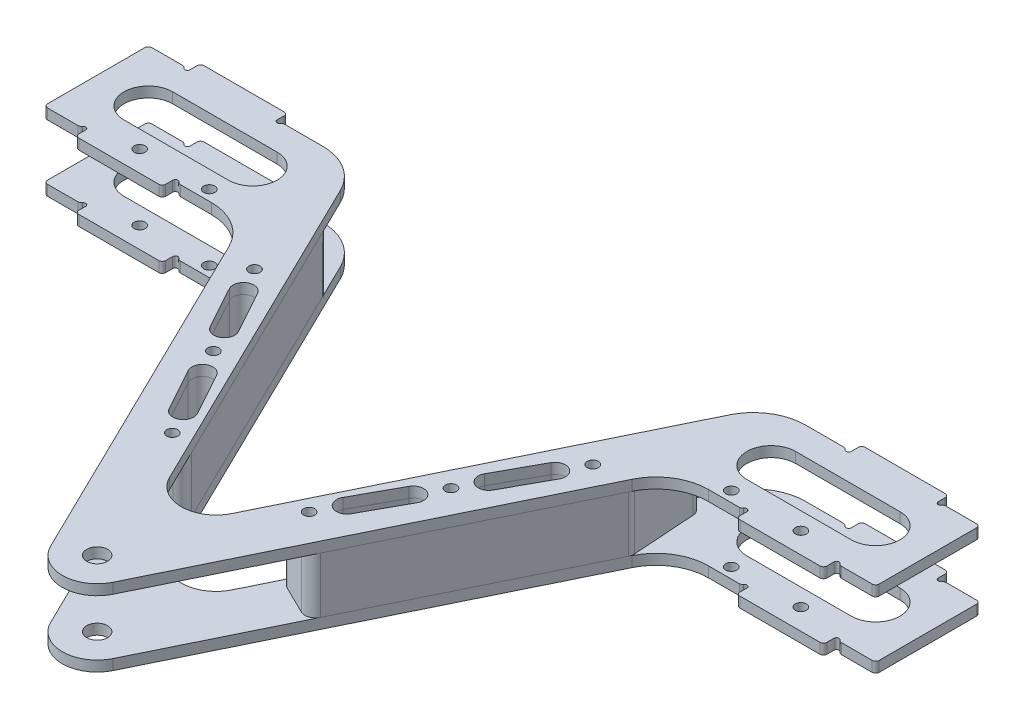
from build123d import *

# Parameters (mm, degrees)
SKETCH_1_R          = 3
EXTRUDE_1_DEPTH     = 3
SKETCH_2_R          = 0.75
CUT_EXTRUDE_1_DEPTH = 3
FILLET_1_R          = 1
EXTRUDE_2_DEPTH     = 16
EXTRUDE_2_2_DEPTH   = 16
SKETCH_4_R          = 1.6
CUT_EXTRUDE_2_DEPTH = 201.908561291
SKETCH_5_R          = 1.6
CUT_EXTRUDE_3_DEPTH = 201.908561291
CUT_EXTRUDE_4_DEPTH = 201.908561291


with BuildPart() as part:
    # 草图1 → 凸台-拉伸1 (new body)
    with BuildSketch(Plane(origin=(0, 0, 0), x_dir=(1, 0, 0), z_dir=(0, 1, 0))):
        with BuildLine():
            Line((-107.5, 127), (-107.5, 124))
            Line((-107.5, 124), (-82.5, 124))
            Line((-82.5, 124), (-82.5, 127))
            Line((-82.5, 127), (-71.405746163, 127))
            ThreePointArc((-71.405746163, 127), (-63.460885028, 124.723174979), (-57.927898376, 118.583890874))
            Line((-57.927898376, 118.583890874), (-8.985231858, 18.393620069))
            ThreePointArc((-8.985231858, 18.393620069), (0, 12.782880651), (8.985231858, 18.393620069))
            Line((8.985231858, 18.393620069), (57.927898376, 118.583890874))
            ThreePointArc((57.927898376, 118.583890874), (63.460885028, 124.723174979), (71.405746163, 127))
            Line((71.405746163, 127), (82.5, 127))
            Line((82.5, 127), (82.5, 124))
            Line((82.5, 124), (107.5, 124))
            Line((107.5, 124), (107.5, 127))
            Line((107.5, 127), (119.5, 127))
            Line((119.5, 127), (119.5, 157))
            Line((119.5, 157), (107.5, 157))
            Line((107.5, 157), (107.5, 160))
            Line((107.5, 160), (82.5, 160))
            Line((82.5, 160), (82.5, 157))
            Line((82.5, 157), (69.366602064, 157))
            ThreePointArc((69.366602064, 157), (61.421740929, 154.723174979), (55.888754277, 148.583890874))
            Line((55.888754277, 148.583890874), (8.985231858, 52.567941045))
            ThreePointArc((8.985231858, 52.567941045), (0, 46.957201628), (-8.985231858, 52.567941045))
            Line((-8.985231858, 52.567941045), (-55.888754277, 148.583890874))
            ThreePointArc((-55.888754277, 148.583890874), (-61.421740929, 154.723174979), (-69.366602064, 157))
            Line((-69.366602064, 157), (-82.5, 157))
            Line((-82.5, 157), (-82.5, 160))
            Line((-82.5, 160), (-107.5, 160))
            Line((-107.5, 160), (-107.5, 157))
            Line((-107.5, 157), (-119.5, 157))
            Line((-119.5, 157), (-119.5, 127))
            Line((-119.5, 127), (-107.5, 127))
        make_face()
        with Locations(Location((0, 22.782880651, 0), (0, 0, 270))):
            Circle(SKETCH_1_R, mode=Mode.SUBTRACT)
    extrude(amount=EXTRUDE_1_DEPTH)

    # 草图2 → 切除-拉伸1 (cut)
    with BuildSketch(Plane(origin=(0, 3, 0), x_dir=(1, 0, 0), z_dir=(0, 1, 0))):
        with Locations((-108.25, 157)):
            Circle(SKETCH_2_R)
        with Locations((-81.75, 157)):
            Circle(SKETCH_2_R)
        with Locations((-108.25, 127)):
            Circle(SKETCH_2_R)
        with Locations((-81.75, 127)):
            Circle(SKETCH_2_R)
        with Locations((81.75, 127)):
            Circle(SKETCH_2_R)
        with Locations((108.25, 127)):
            Circle(SKETCH_2_R)
        with Locations((81.75, 157)):
            Circle(SKETCH_2_R)
        with Locations((108.25, 157)):
            Circle(SKETCH_2_R)
    extrude(amount=-CUT_EXTRUDE_1_DEPTH, mode=Mode.SUBTRACT)

    # 圆角1
    fillet_1_edges = [part.edges().sort_by_distance(p)[0] for p in [
        (81, 1.5, -157),
        (109, 1.5, -127),
        (-81, 1.5, -127),
        (81, 1.5, -127),
        (-109, 1.5, -127),
        (-81, 1.5, -157),
        (109, 1.5, -157),
        (-119.5, 1.5, -127),
        (-119.5, 1.5, -157),
        (-107.5, 1.5, -160),
        (-82.5, 1.5, -160),
        (82.5, 1.5, -160),
        (107.5, 1.5, -160),
        (119.5, 1.5, -157),
        (119.5, 1.5, -127),
        (107.5, 1.5, -124),
        (82.5, 1.5, -124),
        (-82.5, 1.5, -124),
        (-107.5, 1.5, -124),
        (-109, 1.5, -157),
    ]]
    fillet(fillet_1_edges, radius=FILLET_1_R)


with BuildPart() as body_2:
    # 草图3 → 凸台-拉伸2 (new body)
    with BuildSketch(Plane(origin=(0, 3, 0), x_dir=(1, 0, 0), z_dir=(0, 1, 0))):
        with BuildLine():
            Line((-56.650043824, 137.383757235), (-57.873530284, 119.383757235))
            ThreePointArc((-57.873530284, 119.383757235), (-57.824581944, 118.604111022), (-57.576006101, 117.863534079))
            Line((-57.576006101, 117.863534079), (-28.519852473, 58.382837427))
            ThreePointArc((-28.519852473, 58.382837427), (-26.799235652, 56.862457312), (-24.507504741, 57.004046044))
            Line((-24.507504741, 57.004046044), (-16.420796069, 60.954380569))
            ThreePointArc((-16.420796069, 60.954380569), (-14.900415954, 62.674997389), (-15.042004686, 64.966728301))
            Line((-15.042004686, 64.966728301), (-50.961380526, 138.497090429))
            ThreePointArc((-50.961380526, 138.497090429), (-54.233151316, 140.124457655), (-56.650043824, 137.383757235))
        make_face()
    extrude(amount=EXTRUDE_2_DEPTH)


with BuildPart() as body_3:
    # 草图3 → Extrude 2 2 (new body)
    with BuildSketch(Plane(origin=(0, 3, 0), x_dir=(1, 0, 0), z_dir=(0, 1, 0))):
        with BuildLine():
            Line((56.650043824, 137.383757235), (57.873530284, 119.383757235))
            ThreePointArc((57.873530284, 119.383757235), (57.824581944, 118.604111022), (57.576006101, 117.863534079))
            Line((57.576006101, 117.863534079), (28.519852473, 58.382837427))
            ThreePointArc((28.519852473, 58.382837427), (26.799235652, 56.862457312), (24.507504741, 57.004046044))
            Line((24.507504741, 57.004046044), (16.420796069, 60.954380569))
            ThreePointArc((16.420796069, 60.954380569), (14.900415954, 62.674997389), (15.042004686, 64.966728301))
            Line((15.042004686, 64.966728301), (50.961380526, 138.497090429))
            ThreePointArc((50.961380526, 138.497090429), (54.233151316, 140.124457655), (56.650043824, 137.383757235))
        make_face()
    extrude(amount=EXTRUDE_2_2_DEPTH)


with BuildPart() as body_4:
    # 镜向1: mirrored copy
    add(part.part.mirror(Plane.ZX.offset(11)))


with BuildPart() as cut_extrude_2_tool:
    # 草图4 → 切除-拉伸2 (new, through all)
    with BuildSketch(Plane(origin=(0, 22, 0), x_dir=(1, 0, 0), z_dir=(0, 1, 0))):
        with Locations(Location((-48.611834763, 116.600187378, 0), (0, 0, 270))):
            Circle(SKETCH_4_R)
        with Locations(Location((-34.136183253, 90.323667187, 0), (0, 0, 270))):
            Circle(SKETCH_4_R)
        with Locations(Location((-19.660531742, 64.047146996, 0), (0, 0, 270))):
            Circle(SKETCH_4_R)
        with Locations(Location((19.660531742, 64.047146996, 0), (0, 0, 270))):
            Circle(SKETCH_4_R)
        with Locations(Location((34.136183253, 90.323667187, 0), (0, 0, 270))):
            Circle(SKETCH_4_R)
        with Locations(Location((48.611834763, 116.600187378, 0), (0, 0, 270))):
            Circle(SKETCH_4_R)
    extrude(amount=-CUT_EXTRUDE_2_DEPTH)


with BuildPart() as part_1:
    add(part.part)

    # 切除-拉伸2: cut by cut_extrude_2_tool
    add(cut_extrude_2_tool.part, mode=Mode.SUBTRACT)


with BuildPart() as body_2_1:
    add(body_2.part)

    # 切除-拉伸2: cut by cut_extrude_2_tool
    add(cut_extrude_2_tool.part, mode=Mode.SUBTRACT)


with BuildPart() as body_3_1:
    add(body_3.part)

    # 切除-拉伸2: cut by cut_extrude_2_tool
    add(cut_extrude_2_tool.part, mode=Mode.SUBTRACT)


with BuildPart() as body_4_1:
    add(body_4.part)

    # 切除-拉伸2: cut by cut_extrude_2_tool
    add(cut_extrude_2_tool.part, mode=Mode.SUBTRACT)


with BuildPart() as cut_extrude_3_tool:
    # 草图5 → 切除-拉伸3 (new, through all)
    with BuildSketch(Plane(origin=(0, 22, 0), x_dir=(1, 0, 0), z_dir=(0, 1, 0))):
        with Locations(Location((-95, 130, 0), (0, 0, 270))):
            Circle(SKETCH_5_R)
        with Locations(Location((95, 130, 0), (0, 0, 270))):
            Circle(SKETCH_5_R)
        with Locations(Location((-75, 130, 0), (0, 0, 270))):
            Circle(SKETCH_5_R)
        with Locations(Location((75, 130, 0), (0, 0, 270))):
            Circle(SKETCH_5_R)
    extrude(amount=-CUT_EXTRUDE_3_DEPTH)


with BuildPart() as part_2:
    add(part_1.part)

    # 切除-拉伸3: cut by cut_extrude_3_tool
    add(cut_extrude_3_tool.part, mode=Mode.SUBTRACT)


with BuildPart() as body_4_2:
    add(body_4_1.part)

    # 切除-拉伸3: cut by cut_extrude_3_tool
    add(cut_extrude_3_tool.part, mode=Mode.SUBTRACT)


with BuildPart() as cut_extrude_4_tool:
    # 草图6 → 切除-拉伸4 (new, through all)
    with BuildSketch(Plane(origin=(0, 22, 0), x_dir=(1, 0, 0), z_dir=(0, 1, 0))):
        with BuildLine():
            Line((-42.124009008, 111.040680478), (-35.36870497, 98.778304389))
            ThreePointArc((-35.36870497, 98.778304389), (-36.548791838, 94.703087219), (-40.624009008, 95.883174087))
            Line((-40.624009008, 95.883174087), (-47.379313046, 108.145550176))
            ThreePointArc((-47.379313046, 108.145550176), (-46.199226178, 112.220767346), (-42.124009008, 111.040680478))
        make_face()
        with BuildLine():
            Line((42.124009008, 111.040680478), (35.36870497, 98.778304389))
            ThreePointArc((35.36870497, 98.778304389), (36.548791838, 94.703087219), (40.624009008, 95.883174087))
            Line((40.624009008, 95.883174087), (47.379313046, 108.145550176))
            ThreePointArc((47.379313046, 108.145550176), (46.199226178, 112.220767346), (42.124009008, 111.040680478))
        make_face()
        with BuildLine():
            Line((-27.648357498, 84.764160287), (-20.893053459, 72.501784198))
            ThreePointArc((-20.893053459, 72.501784198), (-22.073140328, 68.426567028), (-26.148357498, 69.606653896))
            Line((-26.148357498, 69.606653896), (-32.903661536, 81.869029985))
            ThreePointArc((-32.903661536, 81.869029985), (-31.723574668, 85.944247155), (-27.648357498, 84.764160287))
        make_face()
        with BuildLine():
            Line((27.648357498, 84.764160287), (20.893053459, 72.501784198))
            ThreePointArc((20.893053459, 72.501784198), (22.073140328, 68.426567028), (26.148357498, 69.606653896))
            Line((26.148357498, 69.606653896), (32.903661536, 81.869029985))
            ThreePointArc((32.903661536, 81.869029985), (31.723574668, 85.944247155), (27.648357498, 84.764160287))
        make_face()
        with BuildLine():
            Line((-104.5, 149), (-74.5, 149))
            ThreePointArc((-74.5, 149), (-67.5, 142), (-74.5, 135))
            Line((-74.5, 135), (-104.5, 135))
            ThreePointArc((-104.5, 135), (-111.5, 142), (-104.5, 149))
        make_face()
        with BuildLine():
            Line((104.5, 149), (74.5, 149))
            ThreePointArc((74.5, 149), (67.5, 142), (74.5, 135))
            Line((74.5, 135), (104.5, 135))
            ThreePointArc((104.5, 135), (111.5, 142), (104.5, 149))
        make_face()
    extrude(amount=-CUT_EXTRUDE_4_DEPTH)


with BuildPart() as part_3:
    add(part_2.part)

    # 切除-拉伸4: cut by cut_extrude_4_tool
    add(cut_extrude_4_tool.part, mode=Mode.SUBTRACT)


with BuildPart() as body_2_2:
    add(body_2_1.part)

    # 切除-拉伸4: cut by cut_extrude_4_tool
    add(cut_extrude_4_tool.part, mode=Mode.SUBTRACT)


with BuildPart() as body_3_2:
    add(body_3_1.part)

    # 切除-拉伸4: cut by cut_extrude_4_tool
    add(cut_extrude_4_tool.part, mode=Mode.SUBTRACT)


with BuildPart() as body_4_3:
    add(body_4_2.part)

    # 切除-拉伸4: cut by cut_extrude_4_tool
    add(cut_extrude_4_tool.part, mode=Mode.SUBTRACT)


solid = Compound([part_3.part, body_2_2.part, body_3_2.part, body_4_3.part])
